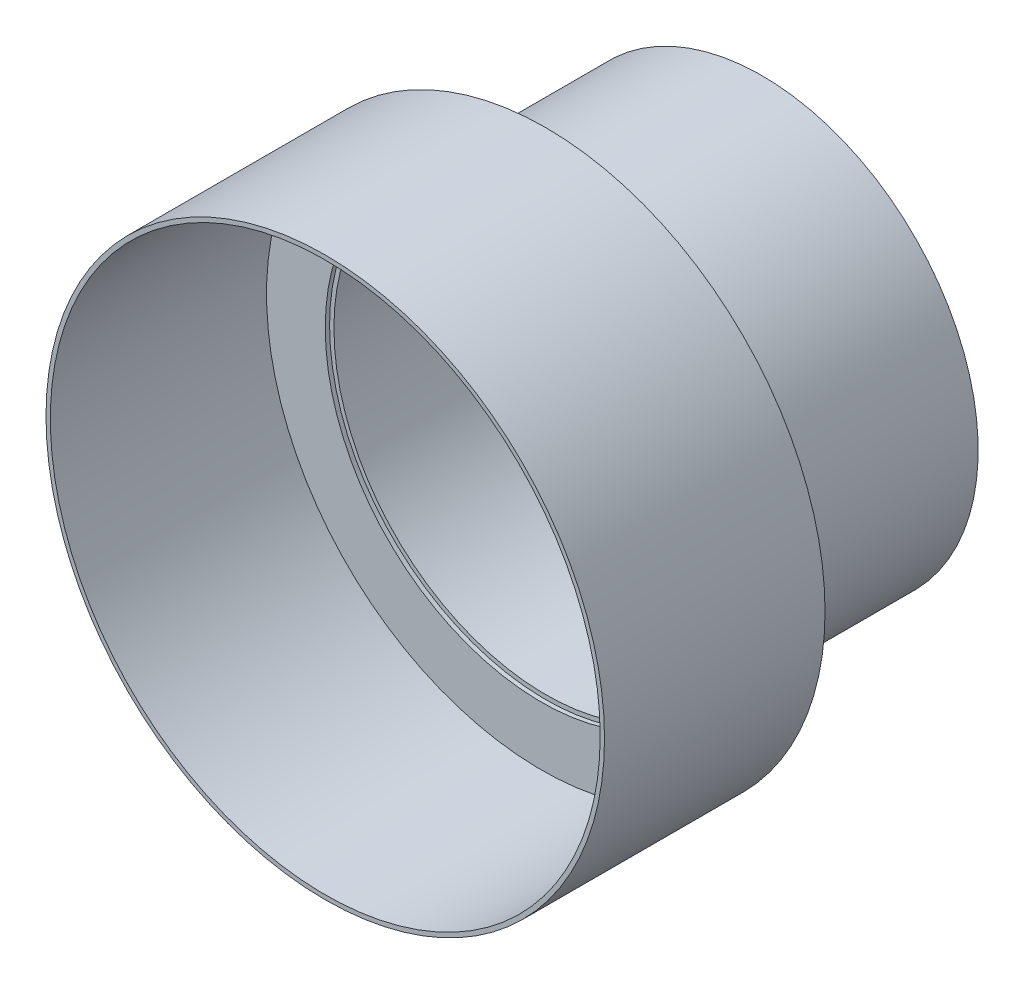
SolidWorks part; units mm, degrees
material "Q235"
ref_plane "Front Plane" through (0, 0, 0) normal (0, 0, 1) x (1, 0, 0)
ref_plane "Top Plane" through (0, 0, 0) normal (0, 1, 0) x (1, 0, 0)
ref_plane "Right Plane" through (0, 0, 0) normal (1, 0, 0) x (0, 0, -1)
sketch "Sketch1" plane through (0, 0, 0) normal (0, 0, 1) x (1, 0, 0)
  circle A0 centre (0, 0) radius 77.5
  circle A1 centre (0, 0) radius 76.3
  dimension "D1" = 1.2
  dimension "D2" = 155
extrude "Boss-Extrude1" add sketch "Sketch1" along normal blind 60
sketch "Sketch2" plane through (0, 0, 0) normal (0, 0, -1) x (-1, 0, 0)
  circle A0 centre (0, 0) radius 60
  circle A1 centre (0, 0) radius 77.5
  circle A2 centre (0, 0) radius 77.5
  dimension "D2" = 120
  dimension "D1" = 0
extrude "Boss-Extrude2" add sketch "Sketch2" along normal blind 1.2
sketch "Sketch3" plane through (0, 0, -1.2) normal (0, 0, -1) x (-1, 0, 0)
  circle A0 centre (0, 0) radius 60 construction
  circle A1 centre (0, 0) radius 60
  circle A2 centre (0, 0) radius 58.8
  dimension "D1" = 1.2
extrude "Boss-Extrude3" add sketch "Sketch3" along normal blind 60 separate body
